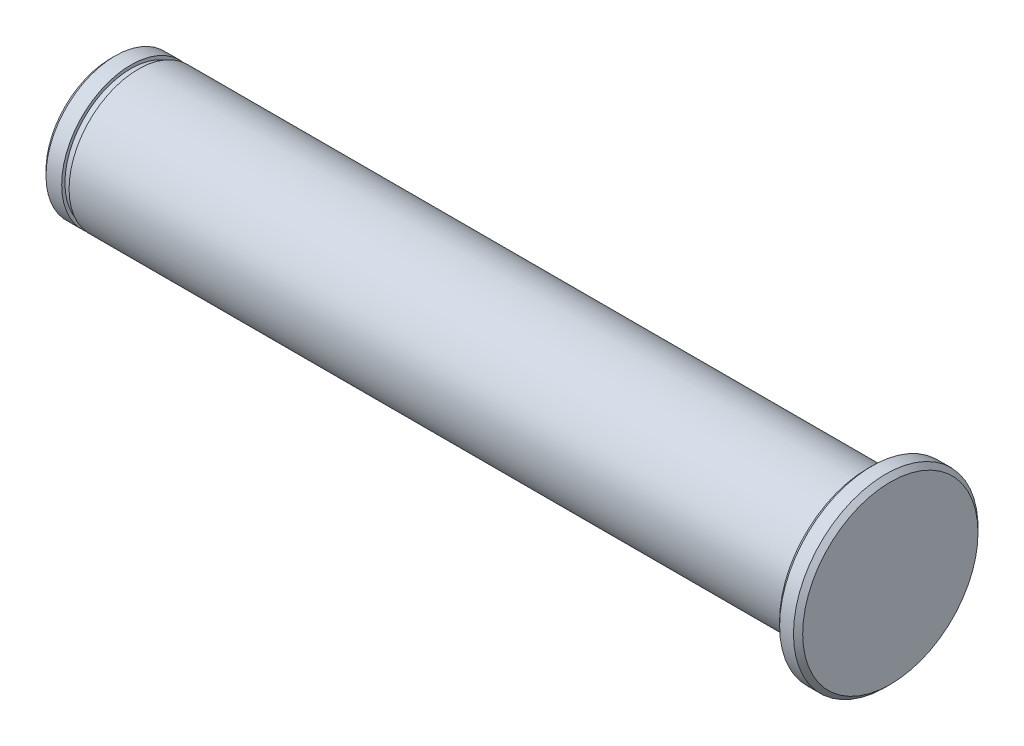
from build123d import *

# Parameters (mm, degrees)
CUT_EXTRUDE_START   = -15
CUT_EXTRUDE_1_DEPTH = 4
CHAMFER_1_SIZE      = 1


with BuildPart() as part:
    # 草图1 → 旋转1 (revolve)
    with BuildSketch(Plane.XY, mode=Mode.PRIVATE) as revolve_1_sk:
        Polygon((0, 0), (0, 15), (4.4, 15), (4.4, 14.3), (6, 14.3), (6, 15), (164, 15), (164, 20), (169, 20), (169, 0), align=None)
    revolve(revolve_1_sk.sketch.rotate(Axis((0, 0, 0), (1, 0, 0)), 90), axis=Axis((0, 0, 0), (1, 0, 0)))

    # 草图2 → 切除-拉伸1 (cut)
    with BuildSketch(Plane.XY.offset(CUT_EXTRUDE_START)):
        with BuildLine():
            Line((119, -4), (49, -4))
            ThreePointArc((49, -4), (45, 0), (49, 4))
            Line((49, 4), (119, 4))
            ThreePointArc((119, 4), (123, 0), (119, -4))
        make_face()
    extrude(amount=CUT_EXTRUDE_1_DEPTH, mode=Mode.SUBTRACT)

    # 倒角1
    chamfer_1_edges = [part.edges().sort_by_distance(p)[0] for p in [
        (0, 0, -15),
        (169, 0, -20),
        (164, 0, -20),
    ]]
    chamfer(chamfer_1_edges, length=CHAMFER_1_SIZE)


solid = part.part
